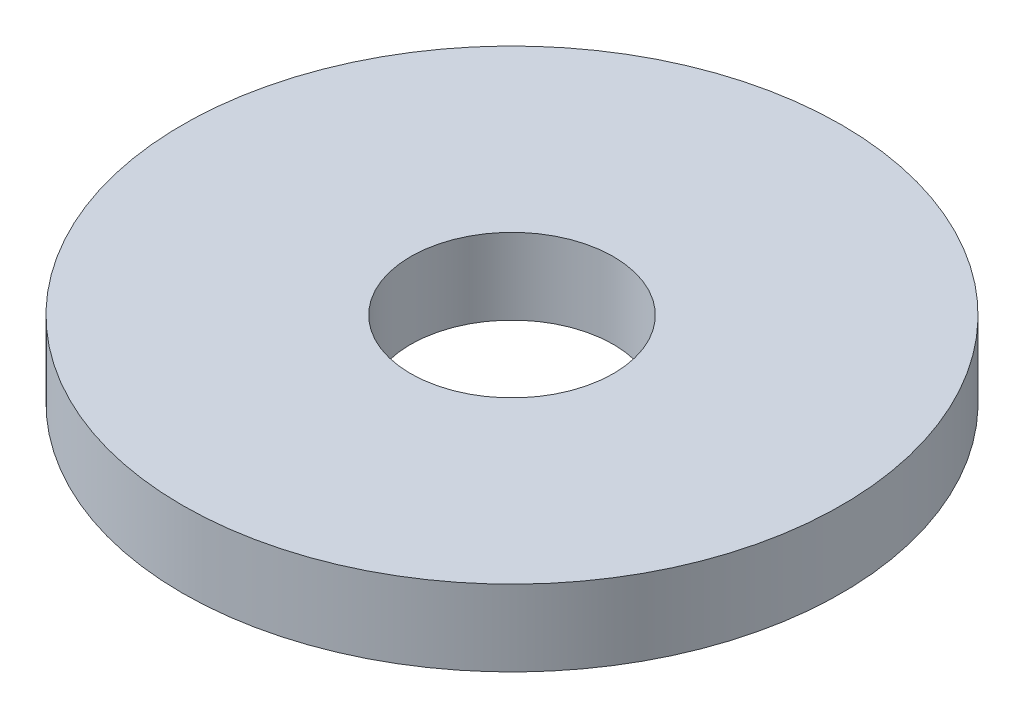
from build123d import *

# Parameters (mm, degrees)
SKETCH_1_R      = 65
SKETCH_1_R_2    = 20
EXTRUDE_1_DEPTH = 7.5


with BuildPart() as part:
    # 草图1 → 凸台-拉伸1 (new, symmetric)
    with BuildSketch(Plane(origin=(0, 0, 0), x_dir=(1, 0, 0), z_dir=(0, 1, 0))):
        with Locations(Location((0, 0, 0), (0, 0, 270))):
            Circle(SKETCH_1_R)
        with Locations(Location((0, 0, 0), (0, 0, 270))):
            Circle(SKETCH_1_R_2, mode=Mode.SUBTRACT)
    extrude(amount=EXTRUDE_1_DEPTH, both=True)


solid = part.part
